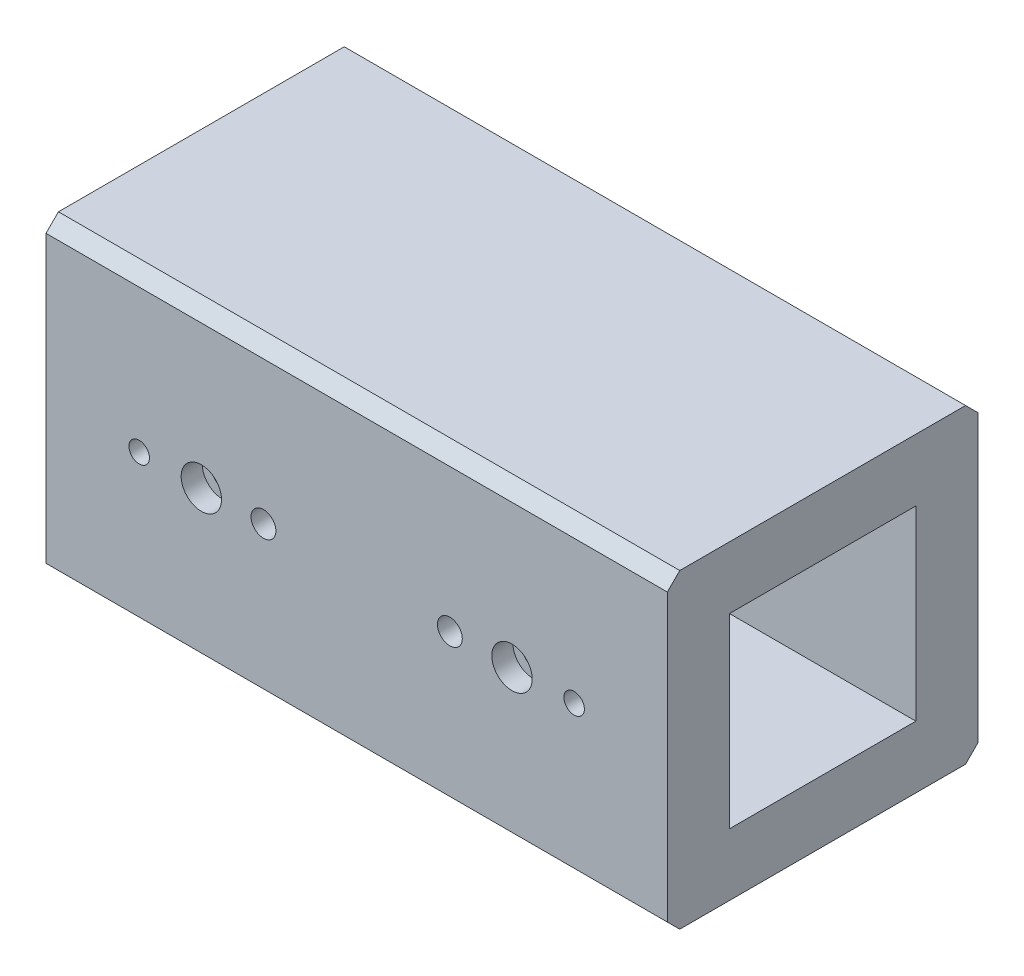
SolidWorks part; units mm, degrees
material "S45C"
ref_plane "Front Plane" through (0, 0, 0) normal (0, 0, 1) x (1, 0, 0)
ref_plane "Top Plane" through (0, 0, 0) normal (0, 1, 0) x (1, 0, 0)
ref_plane "Right Plane" through (0, 0, 0) normal (1, 0, 0) x (0, 0, -1)
sketch "Sketch1" plane through (0, 0, 0) normal (0, 0, 1) x (1, 0, 0)
  line L1 (-50, 25) -> (50, 25)
  line L2 (-50, 25) -> (-50, -25)
  line L3 (-50, -25) -> (50, -25)
  line L4 (50, 25) -> (50, -25)
  line L5 (-50, 25) -> (50, -25) construction
  line L6 (-50, -25) -> (50, 25) construction
  point P0 (0, 0)
  dimension "D1" = 100
  dimension "D2" = 50
extrude "Boss-Extrude1" add sketch "Sketch1" along normal blind 50
sketch "Sketch2" plane through (50, 0, 0) normal (1, 0, 0) x (0, 0, -1)
  line L0 (-50, 25) -> (0, 25) construction
  line L1 (-40, 15) -> (-10, 15)
  line L2 (-40, 15) -> (-40, -15)
  line L3 (-40, -15) -> (-10, -15)
  line L4 (-10, 15) -> (-10, -15)
  line L5 (-50, -25) -> (0, -25) construction
  line L6 (-50, -25) -> (-50, 25) construction
  line L7 (0, -25) -> (0, 25) construction
  dimension "D1" = 10
  dimension "D2" = 10
  dimension "D3" = 10
  dimension "D4" = 10
extrude "Cut-Extrude1" cut sketch "Sketch2" against normal through all
hole_wizard "CBORE for M3 Hex Socket Head Cap Screw1" positions "Sketch4" profile "Sketch3" counterbore size "M3" standard "Iso"
sketch "Sketch4" plane through (0, 0, 0) normal (0, 0, -1) x (-1, 0, 0)
  line L0 (0, 25) -> (0, 0) construction
  line L1 (-50, 25) -> (50, 25) construction
  line L2 (0, 0) -> (-50, 0) construction
  line L3 (-50, -25) -> (-50, 25) construction
  point P0 (-25, 0)
  point P3 (25, 0)
  dimension "D1" = 50
sketch "Sketch3" plane through (25, 0, 0) normal (1, 0, 0) x (0, 1, 0)
  line L0 (0, 0) -> (0, 10)
  line L1 (0, 10) -> (1, 10)
  line L3 (1, 10) -> (1, 3.4)
  line L4 (1, 3.4) -> (3.25, 3.4)
  line L5 (3.25, 3.4) -> (3.25, 0)
  line L7 (3.25, 0) -> (0, 0)
  line L11 (0, -6.35) -> (0, 107.95) construction
  dimension "通孔孔直径" = 2
  dimension "通孔孔深度" = 10
  dimension "柱形沉头孔直径" = 6.5
  dimension "柱形沉头孔深度" = 3.4
hole_wizard "CBORE for M3 Hex Socket Head Cap Screw2" positions "Sketch6" profile "Sketch5" counterbore size "M3" standard "Iso" end condition up to next
sketch "Sketch6" plane through (0, 0, 50) normal (0, 0, 1) x (1, 0, 0)
  line L0 (0, 0) -> (0, 25) construction
  line L1 (50, 25) -> (-50, 25) construction
  line L4 (-50, 0) -> (0, 0) construction
  line L5 (-50, 25) -> (-50, -25) construction
  point P0 (-25, 0)
  point P2 (25, 0)
  dimension "D1" = 50
sketch "Sketch5" plane through (-25, 0, 50) normal (1, 0, 0) x (0, -1, 0)
  line L0 (0, 0) -> (0, 10)
  line L1 (0, 10) -> (1, 10)
  line L3 (1, 10) -> (1, 3.4)
  line L4 (1, 3.4) -> (3.25, 3.4)
  line L5 (3.25, 3.4) -> (3.25, 0)
  line L7 (3.25, 0) -> (0, 0)
  line L11 (0, -6.35) -> (0, 107.95) construction
  dimension "通孔孔直径" = 2
  dimension "通孔孔深度" = 10
  dimension "柱形沉头孔直径" = 6.5
  dimension "柱形沉头孔深度" = 3.4
hole_wizard "M4 Tapped Hole1" positions "Sketch8" profile "Sketch7" tap size "M4" standard "Iso"
sketch "Sketch8" plane through (0, 0, 50) normal (0, 0, 1) x (1, 0, 0)
  line L0 (0, 25) -> (0, 0) construction
  line L1 (50, 25) -> (-50, 25) construction
  line L3 (-50, 0) -> (-35, 0) construction
  line L4 (-50, 25) -> (-50, -25) construction
  point P0 (-35, 0)
  point P2 (35, 0)
  dimension "D1" = 70
sketch "Sketch7" plane through (-35, 0, 50) normal (1, 0, 0) x (0, -1, 0)
  line L0 (0, 0) -> (0, 11.0914)
  line L1 (0, 11.0914) -> (1.65, 10.1)
  line L2 (1.65, 10.1) -> (1.65, 0)
  line L5 (1.65, 0) -> (0, 0)
  line L10 (0, 11.0914) -> (-1.65, 10.1) construction
  line L11 (0, -6.35) -> (0, 107.95) construction
  dimension "螺纹孔钻头直径" = 3.3
  dimension "螺纹孔钻头深度" = 10.1
  dimension "导头角度" = 118
cosmetic thread "Hole thread1" parameters "D1"=8, "D2"=4
cosmetic thread "Hole thread2" parameters "D1"=8, "D2"=4
hole_wizard "Ø4.0 (4) Diameter Hole1" positions "Sketch10" profile "Sketch9" hole size "Ø4.0" standard "Iso"
sketch "Sketch10" plane through (0, 0, 50) normal (0, 0, 1) x (1, 0, 0)
  line L0 (0, 25) -> (0, 0) construction
  line L1 (50, 25) -> (-50, 25) construction
  line L3 (-50, 0) -> (0, 0) construction
  line L4 (-50, 25) -> (-50, -25) construction
  point P0 (15, 0)
  point P2 (-15, 0)
  dimension "D1" = 30
sketch "Sketch9" plane through (15, 0, 50) normal (1, 0, 0) x (0, -1, 0)
  line L0 (0, 0) -> (0, 10)
  line L1 (0, 10) -> (2, 10)
  line L2 (2, 10) -> (2, 0)
  line L5 (2, 0) -> (0, 0)
  line L11 (0, -6.35) -> (0, 107.95) construction
  dimension "通孔孔直径" = 4
  dimension "通孔孔深度" = 10
chamfer "Chamfer1" distance 2 angle 45 4 edges at (0, -25, 50) (0, 25, 50) (0, -25, 0) (0, 25, 0)
hole_wizard "M8 Tapped Hole1" positions "Sketch12" profile "Sketch11" tap size "M8" standard "Iso"
sketch "Sketch12" plane through (0, -25, 0) normal (0, -1, 0) x (-1, 0, 0)
  line L3 (0, -50) -> (0, 0) construction
  line L4 (50, -50) -> (-50, -50) construction
  point P0 (0, -25)
sketch "Sketch11" plane through (0, -25, 25) normal (1, 0, 0) x (0, 0, -1)
  line L0 (0, 0) -> (0, 21.7929)
  line L1 (0, 21.7929) -> (3.4, 19.75)
  line L2 (3.4, 19.75) -> (3.4, 0)
  line L5 (3.4, 0) -> (0, 0)
  line L10 (0, 21.7929) -> (-3.4, 19.75) construction
  line L11 (0, -6.35) -> (0, 107.95) construction
  dimension "螺纹孔钻头直径" = 6.8
  dimension "螺纹孔钻头深度" = 19.75
  dimension "导头角度" = 118
cosmetic thread "Hole thread3" parameters "D1"=10, "D2"=8
hole_wizard "M4 Tapped Hole2" positions "Sketch14" profile "Sketch13" tap size "M4" standard "Iso"
sketch "Sketch14" plane through (0, 0, 3.4) normal (0, 0, -1) x (-1, 0, 0)
  point P0 (-25, 0)
  point P3 (25, 0)
sketch "Sketch13" plane through (25, 0, 3.4) normal (1, 0, 0) x (0, 1, 0)
  line L0 (0, 0) -> (0, 11.0914)
  line L1 (0, 11.0914) -> (1.65, 10.1)
  line L2 (1.65, 10.1) -> (1.65, 0)
  line L5 (1.65, 0) -> (0, 0)
  line L10 (0, 11.0914) -> (-1.65, 10.1) construction
  line L11 (0, -6.35) -> (0, 107.95) construction
  dimension "螺纹孔钻头直径" = 3.3
  dimension "螺纹孔钻头深度" = 10.1
  dimension "导头角度" = 118
cosmetic thread "Hole thread4" parameters "D1"=6.6, "D2"=4
cosmetic thread "Hole thread5" parameters "D1"=6.6, "D2"=4
hole_wizard "M4 Tapped Hole3" positions "Sketch16" profile "Sketch15" tap size "M4" standard "Iso"
sketch "Sketch16" plane through (0, 0, 46.6) normal (0, 0, 1) x (1, 0, 0)
  point P0 (-25, 0)
  point P3 (25, 0)
sketch "Sketch15" plane through (-25, 0, 46.6) normal (1, 0, 0) x (0, -1, 0)
  line L0 (0, 0) -> (0, 11.0914)
  line L1 (0, 11.0914) -> (1.65, 10.1)
  line L2 (1.65, 10.1) -> (1.65, 0)
  line L5 (1.65, 0) -> (0, 0)
  line L10 (0, 11.0914) -> (-1.65, 10.1) construction
  line L11 (0, -6.35) -> (0, 107.95) construction
  dimension "螺纹孔钻头直径" = 3.3
  dimension "螺纹孔钻头深度" = 10.1
  dimension "导头角度" = 118
cosmetic thread "Hole thread6" parameters "D1"=6.6, "D2"=4
cosmetic thread "Hole thread7" parameters "D1"=6.6, "D2"=4
